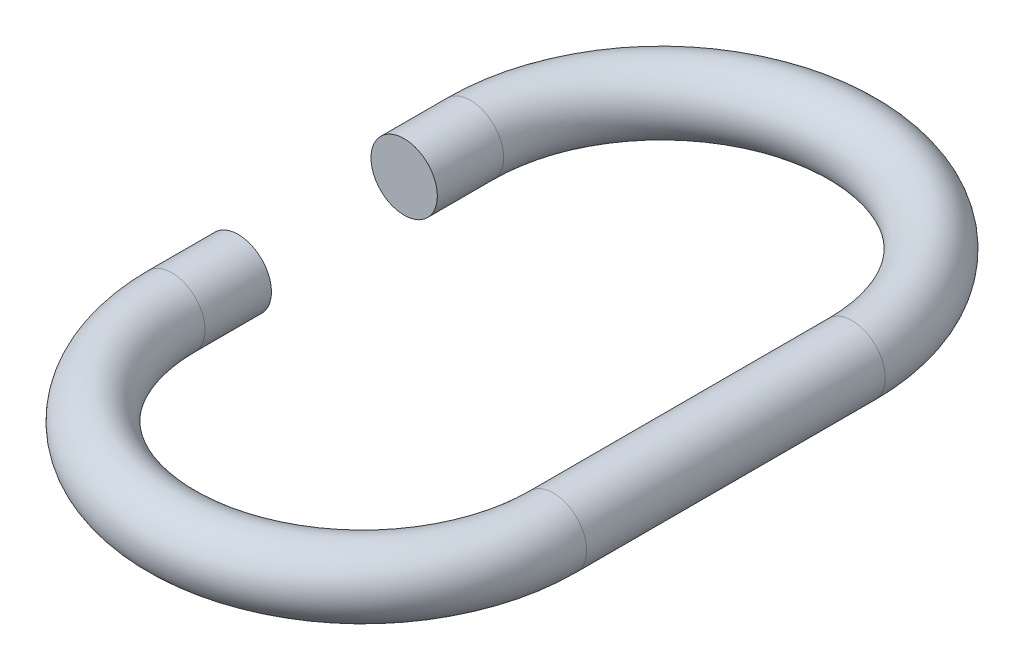
SolidWorks part; units mm, degrees
material "Q235A"
ref_plane "Front Plane" through (0, 0, 0) normal (0, 0, 1) x (1, 0, 0)
ref_plane "Top Plane" through (0, 0, 0) normal (0, 1, 0) x (1, 0, 0)
ref_plane "Right Plane" through (0, 0, 0) normal (1, 0, 0) x (0, 0, -1)
sketch "Sketch1" plane through (0, 0, 0) normal (0, 1, 0) x (1, 0, 0)
  line L0 (-79.6482, 0) -> (65.0243, 0) construction
  line L1 (0, 75.47) -> (0, -65.0243) construction
  line L2 (0, 18) -> (0, -18) construction
  line L3 (23, 18) -> (23, -18)
  line L4 (-23, 18) -> (-23, 10)
  line L8 (-23, -10) -> (-23, -18)
  arc A0 (23, 18) -> (-23, 18) centre (0, 18) ccw
  arc A1 (-23, -18) -> (23, -18) centre (0, -18) ccw
  point P7 (0, 0)
  dimension "D1" = 23
  dimension "D2" = 36
  dimension "D3" = 20
ref_plane "Plane1" through (0, 0, -10) normal (0, 0, 1) x (1, 0, 0)
sketch "Sketch2" plane through (0, 0, -10) normal (0, 0, 1) x (1, 0, 0)
  line L0 (-26.9652, 0) -> (26.719, 0) construction
  circle A0 centre (-23, 0) radius 4
  dimension "D1" = 8
  dimension "D2" = 23
sweep "Sweep1" add profiles "Sketch2" path "Sketch1"
